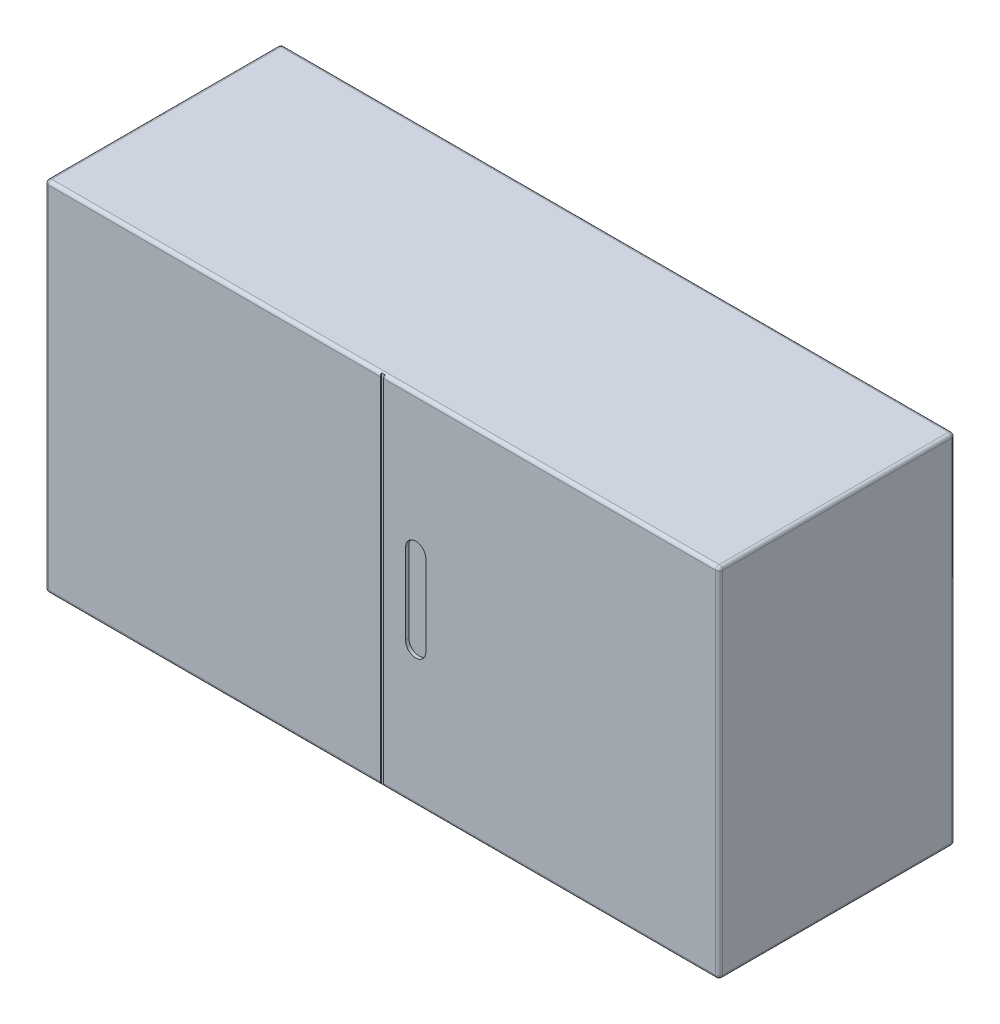
from build123d import *

# Parameters (mm, degrees)
SKETCH1_W           = 1000
SKETCH1_H           = 530
BOSS_EXTRUDE1_DEPTH = 350
FILLET1_R           = 5
SKETCH3_W           = 5
SKETCH3_H           = 530
CUT_EXTRUDE2_DEPTH  = 2
CUT_EXTRUDE3_DEPTH  = 5
SKETCH5_W           = 450
SKETCH5_H           = 60
CUT_EXTRUDE4_DEPTH  = 1
FILLET2_R           = 10


with BuildPart() as part:
    # Sketch1 → Boss-Extrude1 (new body)
    with BuildSketch(Plane.XY):
        Rectangle(SKETCH1_W, SKETCH1_H)
    extrude(amount=BOSS_EXTRUDE1_DEPTH)

    # Fillet1
    fillet1_edges = [part.edges().sort_by_distance(p)[0] for p in [
        (-500, 0, 350),
        (0, -265, 350),
        (500, 0, 350),
        (0, -265, 0),
        (-500, 0, 0),
        (0, 265, 0),
        (500, 0, 0),
        (0, 265, 350),
        (500, -265, 175),
        (-500, -265, 175),
        (-500, 265, 175),
        (500, 265, 175),
    ]]
    fillet(fillet1_edges, radius=FILLET1_R)

    # Sketch3 → Cut-Extrude2 (cut)
    with BuildSketch(Plane.XY.offset(350)):
        Rectangle(SKETCH3_W, SKETCH3_H)
    extrude(amount=-CUT_EXTRUDE2_DEPTH, mode=Mode.SUBTRACT)

    # Sketch4 → Cut-Extrude3 (cut)
    with BuildSketch(Plane.XY.offset(350)):
        with BuildLine():
            Line((65, 60), (65, -60))
            ThreePointArc((65, -60), (50, -75), (35, -60))
            Line((35, -60), (35, 60))
            ThreePointArc((35, 60), (50, 75), (65, 60))
        make_face()
    extrude(amount=-CUT_EXTRUDE3_DEPTH, mode=Mode.SUBTRACT)

    # Sketch5 → Cut-Extrude4 (cut)
    with BuildSketch(Plane.XZ.offset(265)):
        with Locations((0, 175)):
            Rectangle(SKETCH5_W, SKETCH5_H)
    extrude(amount=-CUT_EXTRUDE4_DEPTH, mode=Mode.SUBTRACT)

    # Fillet2
    fillet2_edges = [part.edges().sort_by_distance(p)[0] for p in [
        (225, -264.5, 205),
        (225, -264.5, 145),
        (-225, -264.5, 145),
        (-225, -264.5, 205),
    ]]
    fillet(fillet2_edges, radius=FILLET2_R)


solid = part.part
